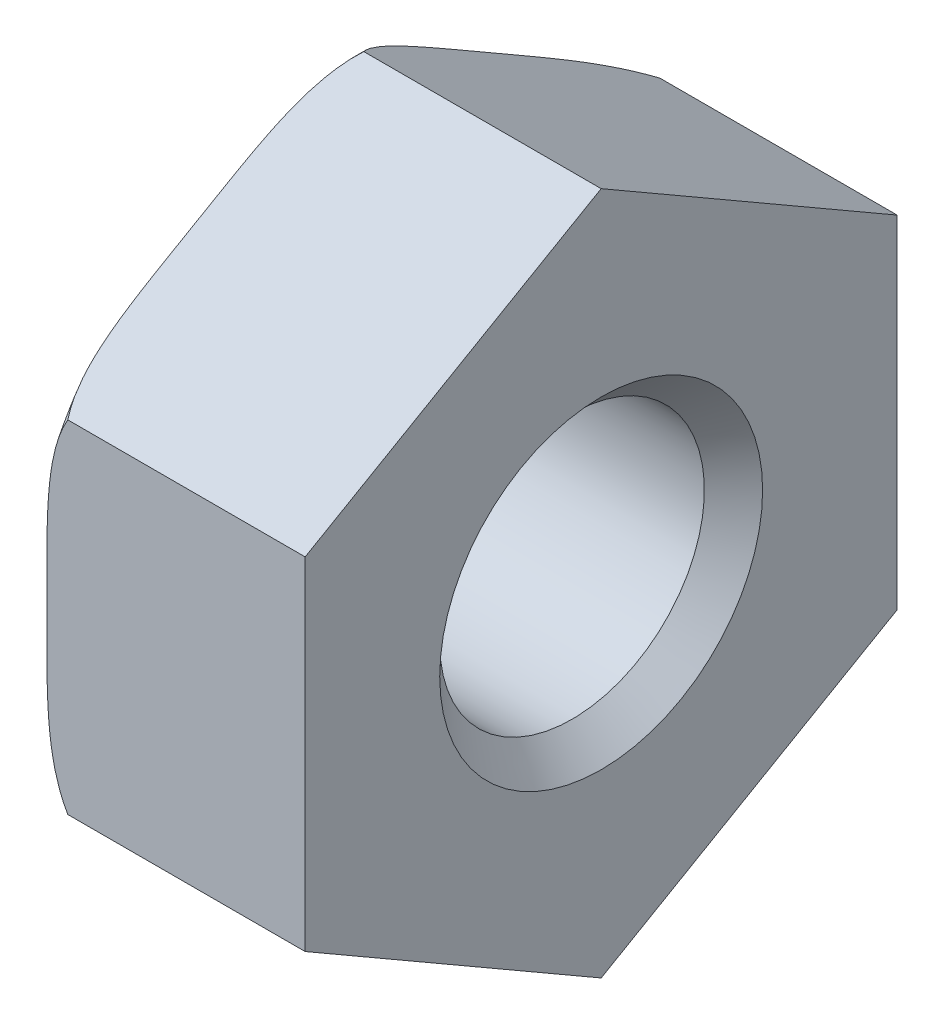
from build123d import *

# Parameters (mm, degrees)
CUT_EXTRUDE1_DEPTH      = 1.2
CUT_EXTRUDE1_DEPTH_BACK = 1.2
SKETCH3_W               = 11
SKETCH3_H               = 11


with BuildPart() as part:
    # Sketch1 → Revolve1 (revolve)
    with BuildSketch(Plane.XY, mode=Mode.PRIVATE) as revolve1_sk:
        with BuildLine():
            Line((-1.2, 0), (-1.2, 2.76))
            ThreePointArc((-1.2, 2.76), (-1.041837662, 3.141837662), (-0.66, 3.3))
            Line((-0.66, 3.3), (1.2, 3.3))
            Line((1.2, 3.3), (1.2, 0))
            Line((1.2, 0), (-1.2, 0))
        make_face()
    revolve(revolve1_sk.sketch.rotate(Axis((1.2, 0, 0), (-1, 0, 0)), 270), axis=Axis((1.2, 0, 0), (-1, 0, 0)))

    # Sketch2 → Cut-Revolve1 (revolve, cut)
    with BuildSketch(Plane.XY, mode=Mode.PRIVATE) as cut_revolve1_sk:
        Polygon((-1.2, 0), (-1.2, 1.5), (-0.9295, 1.2295), (0.9295, 1.2295), (1.2, 1.5), (1.2, 0), align=None)
    revolve(cut_revolve1_sk.sketch.rotate(Axis((1.2, 0, 0), (-1, 0, 0)), 270), axis=Axis((1.2, 0, 0), (-1, 0, 0)), mode=Mode.SUBTRACT)

    # Sketch3 → Cut-Extrude1 (cut, two sides: drawn at the far end of the back side and taken through both)
    with BuildSketch(Plane(origin=(0, 0, 0), x_dir=(0, 0, -1), z_dir=(1, 0, 0)).offset(-CUT_EXTRUDE1_DEPTH_BACK)):
        Rectangle(SKETCH3_W, SKETCH3_H)
        Polygon((-2.75, 1.58771324), (-2.75, -1.58771324), (0, -3.175426481), (2.75, -1.58771324), (2.75, 1.58771324), (0, 3.175426481), align=None, mode=Mode.SUBTRACT)
    extrude(amount=CUT_EXTRUDE1_DEPTH + CUT_EXTRUDE1_DEPTH_BACK, mode=Mode.SUBTRACT)


solid = part.part
